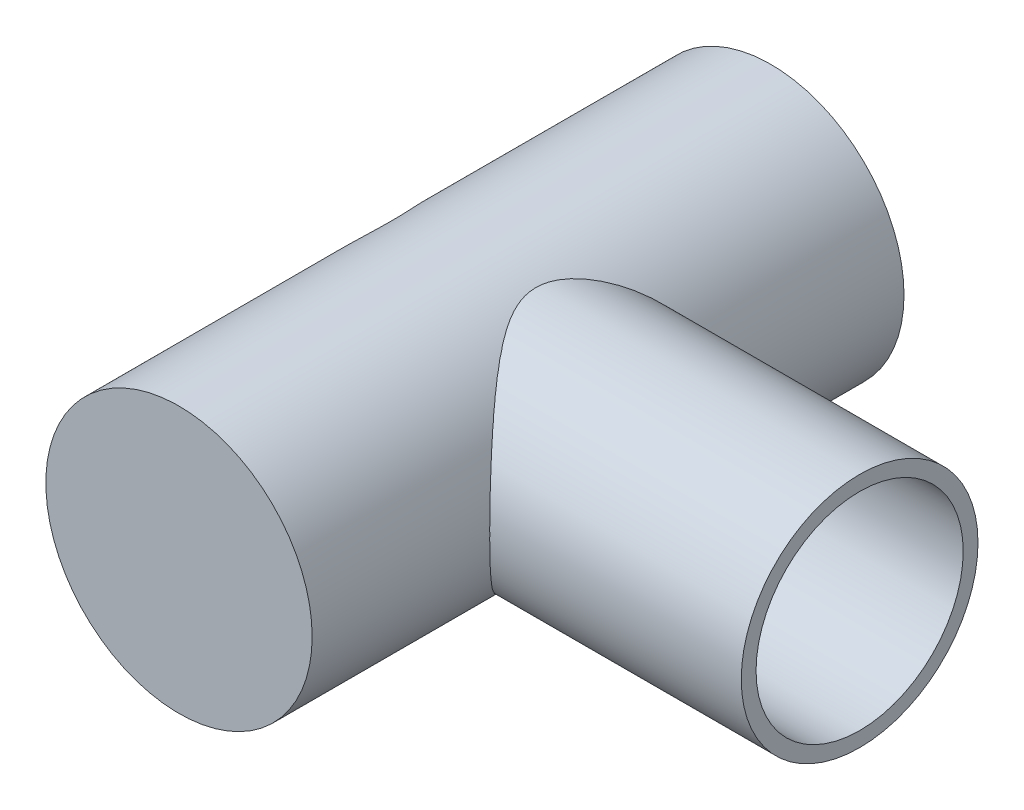
SolidWorks part; units mm, degrees
ref_plane "前视基准面" through (0, 0, 0) normal (0, 0, 1) x (1, 0, 0)
ref_plane "上视基准面" through (0, 0, 0) normal (0, 1, 0) x (1, 0, 0)
ref_plane "右视基准面" through (0, 0, 0) normal (1, 0, 0) x (0, 0, -1)
sketch "草图1" plane through (0, 0, 0) normal (0, 0, 1) x (1, 0, 0)
  circle A0 centre (0, 0) radius 4.5
  dimension "D1" = 9
extrude "凸台-拉伸1" add sketch "草图1" along normal blind 20
ref_plane "基准面1" through (13, 0, 0) normal (1, 0, 0) x (0, 0, -1)
sketch "草图2" plane through (13, 0, 0) normal (1, 0, 0) x (0, 0, -1)
  line L0 (-20, 4.5) -> (-20, -4.5) construction
  circle A0 centre (-10, 0) radius 4
  dimension "D2" = 8
  dimension "D1" = 10
extrude "凸台-拉伸2" add sketch "草图2" against normal up to surface (8.5 mm away) separate body up to face at (4.5, 0, 20)
sketch "草图3" plane through (13, 0, 0) normal (1, 0, 0) x (0, 0, -1)
  circle A0 centre (-10, 0) radius 3.5
  dimension "D1" = 7
extrude "切除-拉伸1" cut sketch "草图3" against normal blind 20
